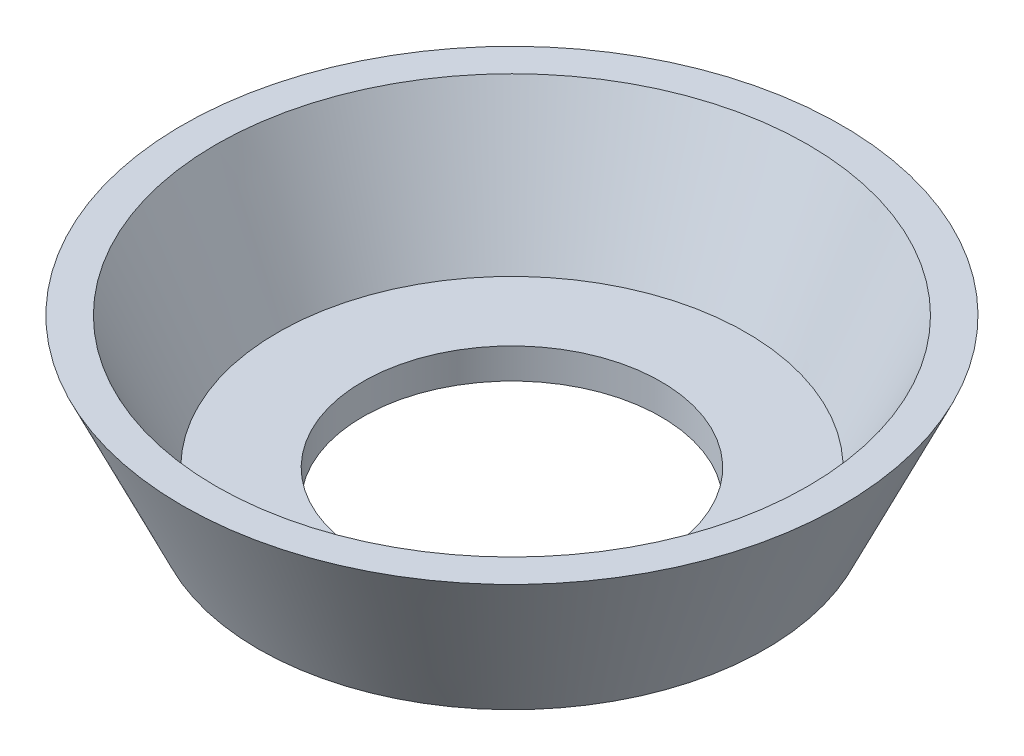
from build123d import *


with BuildPart() as part:
    # 草图1 → 旋转1 (revolve)
    with BuildSketch(Plane.XY, mode=Mode.PRIVATE) as revolve_1_sk:
        Polygon((-32.5, 16), (-25, 0), (-14.7, 0), (-14.7, 3), (-23.093013054, 3), (-29.186763054, 16), align=None)
    revolve(revolve_1_sk.sketch.rotate(Axis((0, 44.007177033, 0), (0, -1, 0)), 270), axis=Axis((0, 44.007177033, 0), (0, -1, 0)))


solid = part.part
